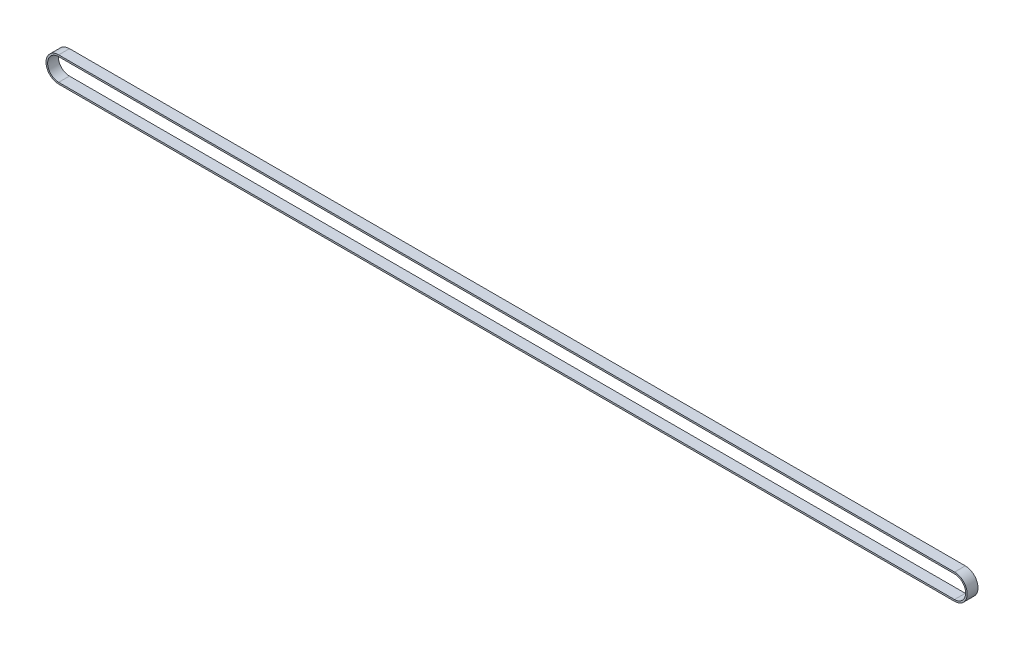
from build123d import *

# Parameters (mm, degrees)
EXTRUDE_1_DEPTH = 30


with BuildPart() as part:
    # 草图1 → 拉伸-薄壁1 (new body)
    with BuildSketch(Plane.XY):
        with BuildLine():
            Line((1246.5, -35.33), (-1246.5, -35.33))
            ThreePointArc((-1246.5, -35.33), (-1281.83, 0), (-1246.5, 35.33))
            Line((-1246.5, 35.33), (1246.5, 35.33))
            ThreePointArc((1246.5, 35.33), (1281.83, 0), (1246.5, -35.33))
        make_face()
        with BuildLine():
            Line((1246.5, -30.83), (-1246.5, -30.83))
            ThreePointArc((-1246.5, -30.83), (-1277.33, 0), (-1246.5, 30.83))
            Line((-1246.5, 30.83), (1246.5, 30.83))
            ThreePointArc((1246.5, 30.83), (1277.33, 0), (1246.5, -30.83))
        make_face(mode=Mode.SUBTRACT)
    extrude(amount=EXTRUDE_1_DEPTH)


solid = part.part
